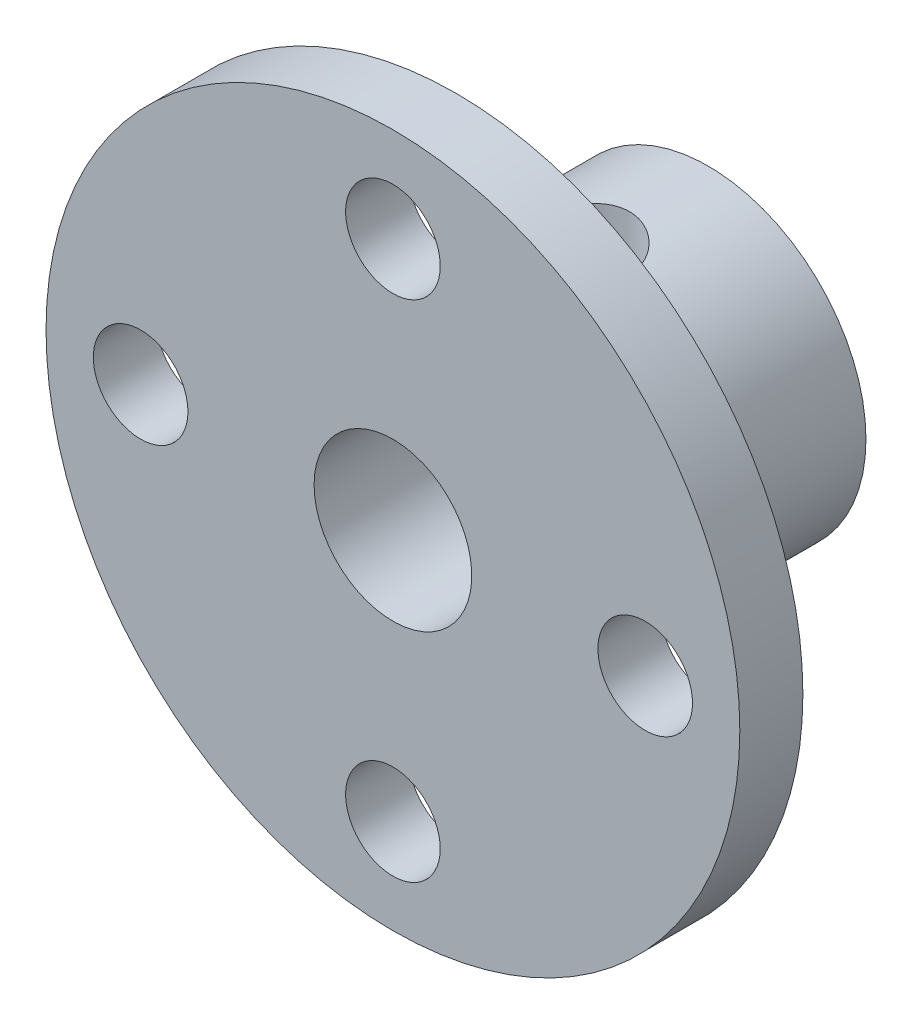
from build123d import *

# Parameters (mm, degrees)
SKETCH1_R           = 11
BOSS_EXTRUDE1_DEPTH = 2
SKETCH2_R           = 5
BOSS_EXTRUDE2_DEPTH = 8
SKETCH3_R           = 2.5
CUT_EXTRUDE1_DEPTH  = 19.493242009
SKETCH4_R           = 1.5
CUT_EXTRUDE2_DEPTH  = 19.493242009
SKETCH5_R           = 1.5
CUT_EXTRUDE3_DEPTH  = 7


with BuildPart() as part:
    # Sketch1 → Boss-Extrude1 (new body)
    with BuildSketch(Plane.XY):
        Circle(SKETCH1_R)
    extrude(amount=BOSS_EXTRUDE1_DEPTH)

    # Sketch2 → Boss-Extrude2 (add)
    with BuildSketch(Plane(origin=(0, 0, 0), x_dir=(-1, 0, 0), z_dir=(0, 0, -1))):
        Circle(SKETCH2_R)
    extrude(amount=BOSS_EXTRUDE2_DEPTH)

    # Sketch3 → Cut-Extrude1 (cut, through all)
    with BuildSketch(Plane(origin=(0, 0, -8), x_dir=(-1, 0, 0), z_dir=(0, 0, -1))):
        Circle(SKETCH3_R)
    extrude(amount=-CUT_EXTRUDE1_DEPTH, mode=Mode.SUBTRACT)

    # Sketch4 → Cut-Extrude2 (cut, through all)
    with BuildSketch(Plane.XY.offset(2)):
        with Locations((0, -8)):
            Circle(SKETCH4_R)
        with Locations((-8, 0)):
            Circle(SKETCH4_R)
        with Locations((0, 8)):
            Circle(SKETCH4_R)
        with Locations((8, 0)):
            Circle(SKETCH4_R)
    extrude(amount=-CUT_EXTRUDE2_DEPTH, mode=Mode.SUBTRACT)

    # Sketch5 → Cut-Extrude3 (cut, symmetric)
    with BuildSketch(Plane(origin=(0, 0, 0), x_dir=(1, 0, 0), z_dir=(0, 1, 0))):
        with Locations(Location((0, 4, 0), (0, 0, 270))):
            Circle(SKETCH5_R)
    extrude(amount=CUT_EXTRUDE3_DEPTH, both=True, mode=Mode.SUBTRACT)


solid = part.part
